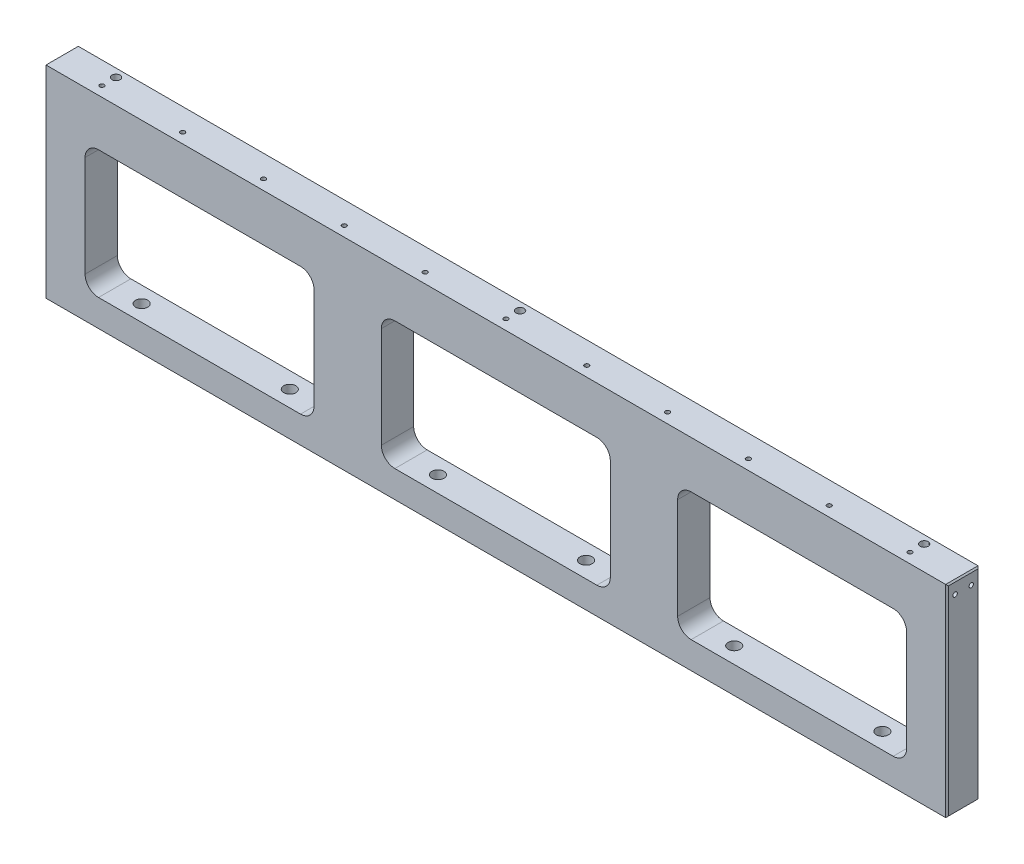
SolidWorks part; units mm, degrees
material "AL6061"
ref_plane "Front View" through (0, 0, 0) normal (0, 0, 1) x (1, 0, 0)
ref_plane "Top View" through (0, 0, 0) normal (0, 1, 0) x (1, 0, 0)
ref_plane "Right View" through (0, 0, 0) normal (1, 0, 0) x (0, 0, -1)
sketch "Sketch1" plane through (0, 0, 0) normal (0, 0, 1) x (1, 0, 0)
  line L1 (-335, -75) -> (335, -75)
  line L2 (-335, -75) -> (-335, 75)
  line L3 (-335, 75) -> (335, 75)
  line L4 (335, -75) -> (335, 75)
  line L5 (-335, -75) -> (335, 75) construction
  line L6 (-335, 75) -> (335, -75) construction
  point P0 (0, 0)
  dimension "D1" = 670
  dimension "D2" = 150
extrude "Boss-Extrude1" add sketch "Sketch1" along normal mid plane 24
sketch "Sketch2" plane through (0, 0, 12) normal (0, 0, 1) x (1, 0, 0)
  line L0 (-335, -75) -> (335, -75) construction
  line L1 (-295, 40) -> (-145, 40)
  line L2 (-305, 30) -> (-305, -45)
  line L3 (-295, -55) -> (-145, -55)
  line L4 (-135, 30) -> (-135, -45)
  line L5 (-335, 75) -> (-335, -75) construction
  line L6 (-75, 40) -> (75, 40)
  line L7 (-85, 30) -> (-85, -45)
  line L8 (-75, -55) -> (75, -55)
  line L9 (85, 30) -> (85, -45)
  line L10 (145, 40) -> (295, 40)
  line L11 (135, 30) -> (135, -45)
  line L12 (145, -55) -> (295, -55)
  line L13 (305, 30) -> (305, -45)
  line L14 (-295, 40) -> (-75, 40) construction
  line L15 (335, -75) -> (335, 75) construction
  line L16 (335, 75) -> (-335, 75) construction
  arc A0 (-305, -45) -> (-295, -55) centre (-295, -45) ccw
  arc A1 (-145, -55) -> (-135, -45) centre (-145, -45) ccw
  arc A2 (-135, 30) -> (-145, 40) centre (-145, 30) ccw
  arc A3 (-295, 40) -> (-305, 30) centre (-295, 30) ccw
  arc A4 (-85, -45) -> (-75, -55) centre (-75, -45) ccw
  arc A5 (75, -55) -> (85, -45) centre (75, -45) ccw
  arc A6 (85, 30) -> (75, 40) centre (75, 30) ccw
  arc A7 (-75, 40) -> (-85, 30) centre (-75, 30) ccw
  arc A8 (135, -45) -> (145, -55) centre (145, -45) ccw
  arc A9 (295, -55) -> (305, -45) centre (295, -45) ccw
  arc A10 (305, 30) -> (295, 40) centre (295, 30) ccw
  arc A11 (145, 40) -> (135, 30) centre (145, 30) ccw
  point P10 (-305, -55)
  point P13 (-135, -55)
  dimension "D5" = 10
  dimension "D1" = 170
  dimension "D2" = 35
  dimension "D3" = 20
  dimension "D4" = 30
  dimension "D7" = 220
  dimension "D8" = 30
  dimension "D6" = 3
extrude "Cut-Extrude1" cut sketch "Sketch2" against normal through all
hole_wizard "M8 Clearance Hole1" positions "Sketch3" profile "Sketch4" hole size "M8" standard "GB"
sketch "Sketch3" plane through (0, -75, 0) normal (0, -1, 0) x (-1, 0, 0)
  line L0 (0, 0) -> (304.414, 0) construction
  line L3 (220, 0) -> (220, -52.9643) construction
  line L6 (305, 12) -> (305, -12) construction
  line L7 (135, 12) -> (135, -12) construction
  line L8 (165, 0) -> (-55, 0) construction
  point P15 (275, 0)
  point P18 (165, 0)
  point P23 (55, 0)
  point P24 (-55, 0)
  point P25 (-165, 0)
  point P26 (-275, 0)
  dimension "D1" = 110
  dimension "D3" = 220
  dimension "D2" = 3
sketch "Sketch4" plane through (275, -75, 0) normal (1, 0, 0) x (0, 0, -1)
  line L0 (0, 0) -> (0, 20)
  line L1 (0, 20) -> (4.5, 20)
  line L2 (4.5, 20) -> (4.5, 0)
  line L5 (4.5, 0) -> (0, 0)
  line L11 (0, -6.35) -> (0, 107.95) construction
  dimension "通孔孔直径" = 9
  dimension "通孔孔深度" = 20
hole_wizard "M4 Tapped Hole1" positions "Sketch5" profile "Sketch6" tap size "M4" standard "GB"
sketch "Sketch5" plane through (0, 75, 0) normal (0, 1, 0) x (1, 0, 0)
  line L0 (-335, -12) -> (-335, 12) construction
  line L1 (335, -12) -> (-335, -12) construction
  line L2 (-300, -4.5) -> (-240, -4.5) construction
  point P0 (-300, -4.5)
  point P11 (-240, -4.5)
  point P12 (-180, -4.5)
  point P13 (-120, -4.5)
  point P14 (-60, -4.5)
  point P15 (0, -4.5)
  point P16 (60, -4.5)
  point P17 (120, -4.5)
  point P18 (180, -4.5)
  point P19 (240, -4.5)
  point P22 (300, -4.5)
  dimension "D1" = 35
  dimension "D2" = 7.5
  dimension "D4" = 60
  dimension "D3" = 11
sketch "Sketch6" plane through (-300, 75, 4.5) normal (1, 0, 0) x (0, 0, 1)
  line L0 (0, 0) -> (0, 11.0914)
  line L1 (0, 11.0914) -> (1.65, 10.1)
  line L2 (1.65, 10.1) -> (1.65, 0)
  line L5 (1.65, 0) -> (0, 0)
  line L10 (0, 11.0914) -> (-1.65, 10.1) construction
  line L11 (0, -6.35) -> (0, 107.95) construction
  dimension "螺纹孔钻头直径" = 3.3
  dimension "螺纹孔钻头深度" = 10.1
  dimension "导头角度" = 118
cosmetic thread "Hole Thread7" parameters "D1"=8, "D2"=4
cosmetic thread "Hole Thread8" parameters "D1"=8, "D2"=4
cosmetic thread "Hole Thread9" parameters "D1"=8, "D2"=4
cosmetic thread "Hole Thread10" parameters "D1"=8, "D2"=4
cosmetic thread "Hole Thread11" parameters "D1"=8, "D2"=4
cosmetic thread "Hole Thread12" parameters "D1"=8, "D2"=4
cosmetic thread "Hole Thread13" parameters "D1"=8, "D2"=4
cosmetic thread "Hole Thread14" parameters "D1"=8, "D2"=4
cosmetic thread "Hole Thread15" parameters "D1"=8, "D2"=4
cosmetic thread "Hole Thread16" parameters "D1"=8, "D2"=4
cosmetic thread "Hole Thread21" parameters "D1"=8, "D2"=4
hole_wizard "Size mm Blind Pin Hole1" positions "Sketch7" profile "Sketch8" hole size "Ø6.0" standard "GB"
sketch "Sketch7" plane through (0, 75, 0) normal (0, 1, 0) x (1, 0, 0)
  line L0 (-300, -4.5) -> (-300, 14.7507) construction
  line L1 (-300, 6) -> (0, 6) construction
  circle A0 centre (-300, -4.5) radius 1.65 construction
  point P8 (-300, 6)
  point P17 (0, 6)
  point P18 (300, 6)
  dimension "D1" = 10.5
  dimension "D3" = 300
  dimension "D2" = 3
sketch "Sketch8" plane through (300, 75, -6) normal (1, 0, 0) x (0, 0, 1)
  line L0 (0, 0) -> (0, 11.9026)
  line L1 (0, 11.9026) -> (3, 10.1)
  line L2 (3, 10.1) -> (3, 0)
  line L5 (3, 0) -> (0, 0)
  line L10 (0, 11.9026) -> (-3, 10.1) construction
  line L11 (0, -6.35) -> (0, 107.95) construction
  dimension "孔直径" = 6
  dimension "孔深度" = 10.1
  dimension "导头角度" = 118
chamfer "Chamfer1" distance 1 angle 45 8 edges at (-335, 75, 0) (-335, 0, 12) (-335, -75, 0) (-335, 0, -12) (335, -75, 0) (335, 0, 12) (335, 75, 0) (335, 0, -12)
hole_wizard "M4 Tapped Hole2" positions "Sketch9" profile "Sketch10" tap size "M4" standard "GB"
sketch "Sketch9" plane through (335, 0, 0) normal (1, 0, 0) x (0, 0, -1)
  line L0 (0, 0) -> (0, 94.0584) construction
  line L1 (-12, 75) -> (12, 75) construction
  point P7 (-6, 66)
  point P10 (6, 66)
  dimension "D1" = 12
  dimension "D2" = 9
sketch "Sketch10" plane through (335, 66, -6) normal (0, 1, 0) x (0, 0, -1)
  line L0 (0, 0) -> (0, 11.0914)
  line L1 (0, 11.0914) -> (1.65, 10.1)
  line L2 (1.65, 10.1) -> (1.65, 0)
  line L5 (1.65, 0) -> (0, 0)
  line L10 (0, 11.0914) -> (-1.65, 10.1) construction
  line L11 (0, -6.35) -> (0, 107.95) construction
  dimension "螺纹孔钻头直径" = 3.3
  dimension "螺纹孔钻头深度" = 10.1
  dimension "导头角度" = 118
cosmetic thread "Hole Thread17" parameters "D1"=8, "D2"=4
cosmetic thread "Hole Thread18" parameters "D1"=8, "D2"=4
hole_wizard "M4 Tapped Hole3" positions "Sketch11" profile "Sketch12" tap size "M4" standard "GB"
sketch "Sketch11" plane through (-335, 0, 0) normal (-1, 0, 0) x (0, 0, 1)
  point P0 (-6, 66)
  point P3 (6, 66)
sketch "Sketch12" plane through (-335, 66, -6) normal (0, 1, 0) x (0, 0, 1)
  line L0 (0, 0) -> (0, 11.0914)
  line L1 (0, 11.0914) -> (1.65, 10.1)
  line L2 (1.65, 10.1) -> (1.65, 0)
  line L5 (1.65, 0) -> (0, 0)
  line L10 (0, 11.0914) -> (-1.65, 10.1) construction
  line L11 (0, -6.35) -> (0, 107.95) construction
  dimension "螺纹孔钻头直径" = 3.3
  dimension "螺纹孔钻头深度" = 10.1
  dimension "导头角度" = 118
cosmetic thread "Hole Thread19" parameters "D1"=8, "D2"=4
cosmetic thread "Hole Thread20" parameters "D1"=8, "D2"=4
hole_wizard "M3 Tapped Hole1" positions "Sketch13" profile "Sketch14" tap size "M3" standard "ISO"
sketch "Sketch13" plane through (0, 0, -12) normal (0, 0, 1) x (1, 0, 0)
  line L0 (0, 0) -> (0, 166.7652) construction
  line L3 (-363.5313, 59) -> (364.2018, 59) construction
  line L6 (-305, 95.4925) -> (-305, -37.1408) construction
  line L9 (334, 75) -> (-334, 75) construction
  line L10 (305, 95.4925) -> (305, -37.1408) construction
  line L11 (-335, -74) -> (-335, 74) construction
  point P19 (-314.85, 59)
  point P22 (-295.15, 59)
  point P25 (295.15, 59)
  point P26 (314.85, 59)
  dimension "D1" = 16
  dimension "D2" = 19.7
  dimension "D3" = 30
sketch "Sketch14" plane through (314.85, 59, -12) normal (1, 0, 0) x (0, 1, 0)
  line L0 (0, 0) -> (0, 8.2511)
  line L1 (0, 8.2511) -> (1.25, 7.5)
  line L2 (1.25, 7.5) -> (1.25, 0)
  line L5 (1.25, 0) -> (0, 0)
  line L10 (0, 8.2511) -> (-1.25, 7.5) construction
  line L11 (0, -6.35) -> (0, 107.95) construction
  dimension "螺纹孔钻头直径" = 2.5
  dimension "螺纹孔钻头深度" = 7.5
  dimension "导头角度" = 118
cosmetic thread "Hole Thread22" parameters "D1"=6, "D2"=3
cosmetic thread "Hole Thread23" parameters "D1"=6, "D2"=3
cosmetic thread "Hole Thread24" parameters "D1"=6, "D2"=3
cosmetic thread "Hole Thread25" parameters "D1"=6, "D2"=3
hole_wizard "M4 Tapped Hole4" positions "Sketch15" profile "Sketch16" tap size "M4" standard "ISO"
sketch "Sketch15" plane through (0, 0, -12) normal (0, 0, -1) x (-1, 0, 0)
  line L0 (109, 75) -> (109, -13.1813) construction
  line L1 (-334, 75) -> (334, 75) construction
  line L4 (63.9958, 55) -> (146.8956, 55) construction
  line L7 (85, 30) -> (85, -45) construction
  point P16 (109, 47.5)
  point P19 (109, 62.5)
  dimension "D1" = 20
  dimension "D2" = 24
  dimension "D3" = 15
sketch "Sketch16" plane through (-109, 62.5, -12) normal (1, 0, 0) x (0, 1, 0)
  line L0 (0, 0) -> (0, 11.0914)
  line L1 (0, 11.0914) -> (1.65, 10.1)
  line L2 (1.65, 10.1) -> (1.65, 0)
  line L5 (1.65, 0) -> (0, 0)
  line L10 (0, 11.0914) -> (-1.65, 10.1) construction
  line L11 (0, -6.35) -> (0, 107.95) construction
  dimension "螺纹孔钻头直径" = 3.3
  dimension "螺纹孔钻头深度" = 10.1
  dimension "导头角度" = 118
cosmetic thread "Hole Thread26" parameters "D1"=8, "D2"=4
cosmetic thread "Hole Thread27" parameters "D1"=8, "D2"=4
